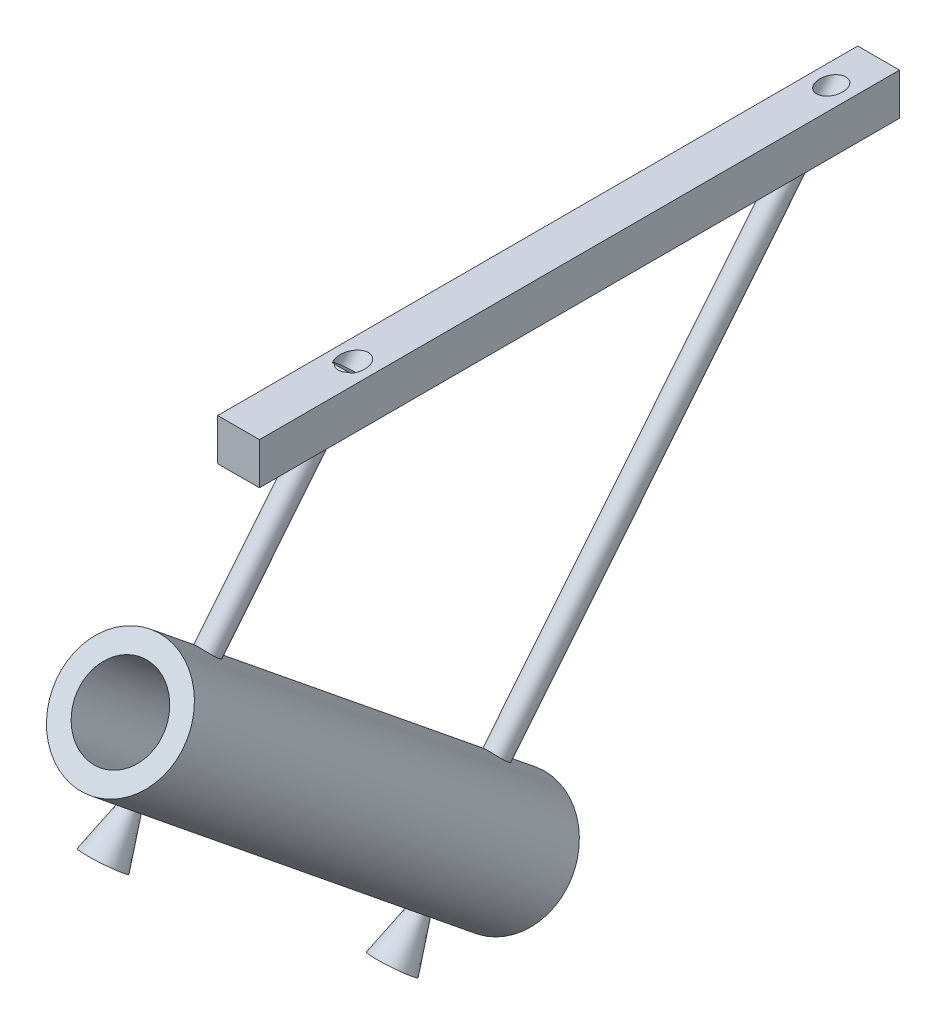
from build123d import *

# Parameters (mm, degrees)
SKETCH2_W                     = 15
SKETCH2_H                     = 230
BOSS_EXTRUDE2_DEPTH           = 15
SKETCH4_R                     = 4
BOSS_EXTRUDE3_DEPTH           = 155
SKETCH5_R                     = 4.473763718
CUT_EXTRUDE1_DEPTH            = 120
SKETCH6_R                     = 4.1
CUT_EXTRUDE2_DEPTH            = 17
SKETCH7_R                     = 5.311376806
SKETCH7_R_2                   = 5.6699774
CUT_EXTRUDE3_DEPTH            = 62
SKETCH8_R                     = 22.5
BOSS_EXTRUDE4_DEPTH           = 178
SKETCH9_R                     = 4.2
CUT_EXTRUDE4_DEPTH            = 8
SKETCH10_R                    = 2
BOSS_EXTRUDE5_DEPTH           = 20
BOSS_EXTRUDE5_DRAFT           = -15
BOSS_EXTRUDE5_PROFILE_2_DEPTH = 20
BOSS_EXTRUDE5_PROFILE_2_DRAFT = -15
SKETCH11_R                    = 15
CUT_EXTRUDE5_DEPTH            = 193


with BuildPart() as part:
    # Sketch2 → Boss-Extrude2 (new body)
    with BuildSketch(Plane(origin=(0, 0, 0), x_dir=(1, 0, 0), z_dir=(0, 1, 0))):
        with Locations((-7.5, -115)):
            Rectangle(SKETCH2_W, SKETCH2_H)
    extrude(amount=BOSS_EXTRUDE2_DEPTH)

    # Sketch4 → Boss-Extrude3 (add, symmetric)
    with BuildSketch(Plane(origin=(0, -112.486974084, 91.090155556), x_dir=(1, 0, 0), z_dir=(0, 0.7771459614569742, -0.6293203910498333))):
        with Locations(Location((-7.5, -22.665437835, 0), (0, 0, 270))):
            Circle(SKETCH4_R)
        with Locations(Location((-7.5, -156.375872868, 0), (0, 0, 270))):
            Circle(SKETCH4_R)
    extrude(amount=BOSS_EXTRUDE3_DEPTH, both=True)

    # Sketch5 → Cut-Extrude1 (cut)
    with BuildSketch(Plane(origin=(0, 7.970649941, -6.454505057), x_dir=(1, 0, 0), z_dir=(0, 0.7771459614569743, -0.6293203910498333))):
        with Locations((-7.5, -156.375872868)):
            Circle(SKETCH5_R)
    extrude(amount=-CUT_EXTRUDE1_DEPTH, mode=Mode.SUBTRACT)

    # Sketch6 → Cut-Extrude2 (cut)
    with BuildSketch(Plane(origin=(0, 7.970649941, -6.454505057), x_dir=(1, 0, 0), z_dir=(0, 0.7771459614569743, -0.6293203910498333))):
        with Locations(Location((-7.5, -22.665437835, 0), (0, 0, 270))):
            Circle(SKETCH6_R)
    extrude(amount=-CUT_EXTRUDE2_DEPTH, mode=Mode.SUBTRACT)

    # Sketch7 → Cut-Extrude3 (cut)
    with BuildSketch(Plane(origin=(0, -232.94459811, 188.634816169), x_dir=(1, 0, 0), z_dir=(0, -0.7771459614569743, 0.6293203910498333))):
        with Locations((-7.5, 22.665437835)):
            Circle(SKETCH7_R)
        with Locations((-7.5, 156.375872868)):
            Circle(SKETCH7_R_2)
    extrude(amount=-CUT_EXTRUDE3_DEPTH, mode=Mode.SUBTRACT)

    # Sketch8 → Boss-Extrude4 (add)
    with BuildSketch(Plane(origin=(0, 112.486974084, 138.909844444), x_dir=(1, 0, 0), z_dir=(0, -0.6293203910498333, -0.7771459614569743))):
        with Locations(Location((-7.5, 212.198540139, 0), (0, 0, 270))):
            Circle(SKETCH8_R)
    extrude(amount=BOSS_EXTRUDE4_DEPTH)

    # Sketch9 → Cut-Extrude4 (cut)
    with BuildSketch(Plane(origin=(0, -184.7615485, 149.616951924), x_dir=(1, 0, 0), z_dir=(0, -0.7771459614569743, 0.6293203910498334))):
        with Locations(Location((-7.5, 156.375872868, 0), (0, 0, 270))):
            Circle(SKETCH9_R)
        with Locations(Location((-7.5, 22.665437835, 0), (0, 0, 270))):
            Circle(SKETCH9_R)
    extrude(amount=-CUT_EXTRUDE4_DEPTH, mode=Mode.SUBTRACT)


with BuildPart() as boss_extrude5_tool:
    # Sketch10 → Boss-Extrude5 (with draft: the straight prism first)
    with BuildSketch(Plane(origin=(0, -178.544380808, 144.582388795), x_dir=(1, 0, 0), z_dir=(0, -0.777145961456974, 0.6293203910498335))):
        with Locations((-7.5, 156.375872868)):
            Circle(SKETCH10_R)
    extrude(amount=BOSS_EXTRUDE5_DEPTH)
    # Boss-Extrude5: the draft: its side faces are tilted about the plane it starts from
    boss_extrude5_sides = [boss_extrude5_tool.faces().sort_by_distance(p)[0] for p in [
        (-9.5, -87.905314959, 272.402470774),
    ]]
    draft(boss_extrude5_sides, Plane(origin=(0, -178.544380808, 144.582388795), x_dir=(1, 0, 0), z_dir=(0, -0.777145961456974, 0.6293203910498335)), BOSS_EXTRUDE5_DRAFT)


with BuildPart() as part_1:
    add(part.part)

    # Boss-Extrude5: add boss_extrude5_tool
    add(boss_extrude5_tool.part)


with BuildPart() as boss_extrude5_profile_2_tool:
    # Sketch10 → Boss-Extrude5 profile 2 (with draft: the straight prism first)
    with BuildSketch(Plane(origin=(0, -178.544380808, 144.582388795), x_dir=(1, 0, 0), z_dir=(0, -0.777145961456974, 0.6293203910498335))):
        with Locations((-7.5, 22.665437835)):
            Circle(SKETCH10_R)
    extrude(amount=BOSS_EXTRUDE5_PROFILE_2_DEPTH)
    # Boss-Extrude5 profile 2: the draft: its side faces are tilted about the plane it starts from
    boss_extrude5_profile_2_sides = [boss_extrude5_profile_2_tool.faces().sort_by_distance(p)[0] for p in [
        (-9.5, -172.052018221, 168.489946184),
    ]]
    draft(boss_extrude5_profile_2_sides, Plane(origin=(0, -178.544380808, 144.582388795), x_dir=(1, 0, 0), z_dir=(0, -0.777145961456974, 0.6293203910498335)), BOSS_EXTRUDE5_PROFILE_2_DRAFT)


with BuildPart() as part_2:
    add(part_1.part)

    # Boss-Extrude5 profile 2: add boss_extrude5_profile_2_tool
    add(boss_extrude5_profile_2_tool.part)

    # Sketch11 → Cut-Extrude5 (cut)
    with BuildSketch(Plane(origin=(0, 112.486974084, 138.909844444), x_dir=(1, 0, 0), z_dir=(0, 0.6293203910498334, 0.7771459614569743))):
        with Locations(Location((-7.5, -212.198540139, 0), (0, 0, 270))):
            Circle(SKETCH11_R)
    extrude(amount=-CUT_EXTRUDE5_DEPTH, mode=Mode.SUBTRACT)


solid = part_2.part
